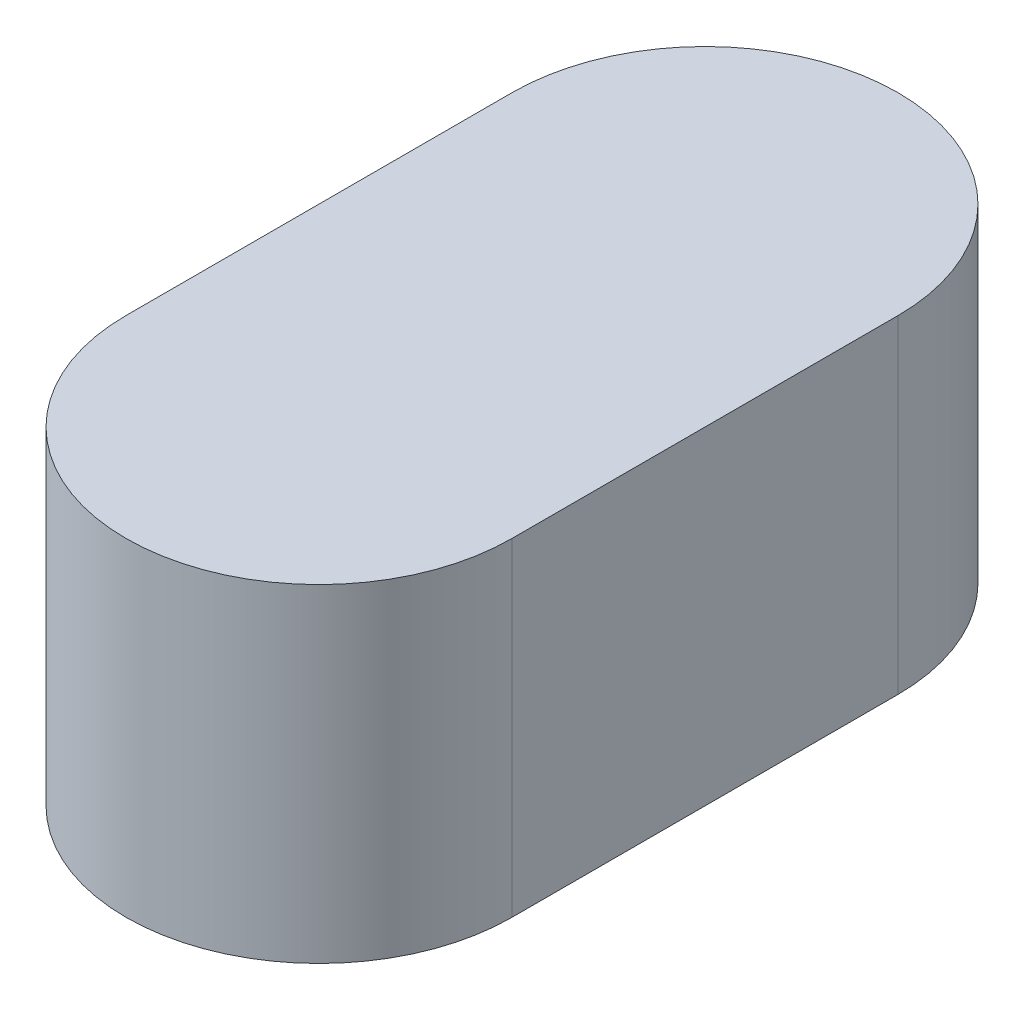
from build123d import *

# Parameters (mm, degrees)
BOSS_EXTRUDE1_DEPTH = 8.5


with BuildPart() as part:
    # Sketch1 → Boss-Extrude1 (new body)
    with BuildSketch(Plane(origin=(0, 0, 0), x_dir=(1, 0, 0), z_dir=(0, 1, 0))):
        with BuildLine():
            Line((-5, 5), (-5, -5))
            ThreePointArc((-5, -5), (0, -10), (5, -5))
            Line((5, -5), (5, 5))
            ThreePointArc((5, 5), (0, 10), (-5, 5))
        make_face()
    extrude(amount=BOSS_EXTRUDE1_DEPTH)


solid = part.part
